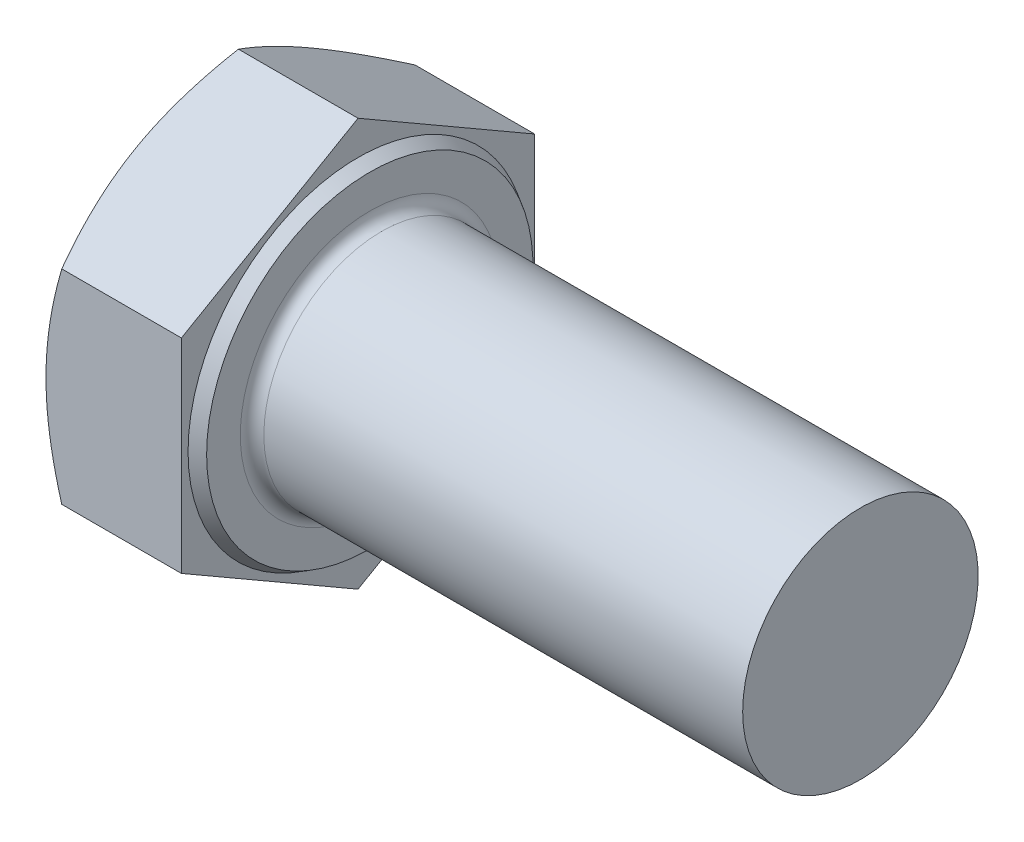
SolidWorks part; units mm, degrees
ref_plane "前视" through (0, 0, 0) normal (0, 0, 1) x (1, 0, 0)
ref_plane "上视" through (0, 0, 0) normal (0, 1, 0) x (1, 0, 0)
ref_plane "右视" through (0, 0, 0) normal (1, 0, 0) x (0, 0, -1)
sketch "草图1" plane through (0, 0, 0) normal (1, 0, 0) x (0, 0, -1)
  line L0 (9, 5.1962) -> (9, -5.1962)
  line L1 (-9, 5.1962) -> (-9, -5.1962)
  line L2 (9, -5.1962) -> (0, -10.3923)
  line L3 (0, -10.3923) -> (-9, -5.1962)
  line L4 (9, 5.1962) -> (0, 10.3923)
  line L5 (0, 10.3923) -> (-9, 5.1962)
  circle A0 centre (0, 0) radius 10.015 construction
  dimension "e" = 20.03
  dimension "s" = 18
  dimension "D2" = 120
  dimension "D3" = 9
  dimension "D4" = 9
  dimension "D5" = 9
extrude "基体-拉伸" add sketch "草图1" along normal blind 7.5
sketch "草图2" plane through (0, 0, 0) normal (0, 0, 1) x (1, 0, 0)
  line L0 (0, 5.1962) -> (0, -5.1962) construction
  line L1 (0, 0) -> (32.5, 0)
  line L2 (0, 0) -> (0, 6)
  line L3 (0, 6) -> (2.5, 6)
  line L4 (32.5, 0) -> (32.5, 4.4845)
  line L5 (7.5, 10.3923) -> (7.5, 5.1962) construction
  line L7 (0, 0) -> (44.5, 0) construction
  line L8 (32.5, -4.4845) -> (2.5, -6) construction
  line L9 (0, -6) -> (2.5, -6) construction
  line L10 (9.25, 6) -> (9.25, 0) construction
  line L11 (2.5, 15.24) -> (2.5, -1.27) construction
  line L12 (7.5, 5.1962) -> (7.5, -5.1962) construction
  line L13 (2.5, 6) -> (32.5, 6)
  line L14 (32.5, 6) -> (32.5, 4.4845)
  dimension "l" = 25
  dimension "d" = 12
  dimension "Minor_dia" = 8.969
  dimension "p" = 1.75
  dimension "b" = 30
  dimension "ds" = 12
revolve "凸台-旋转1" add sketch "草图2" angle 360 about L7
cosmetic thread "螺旋线1" parameters "Thread_length"=30, "Thread_minor"=8.969
sketch "草图3" plane through (0, 0, 0) normal (0, 0, 1) x (1, 0, 0)
  line L0 (0, 9) -> (3.6906, 15.3923)
  line L1 (0, 10.3923) -> (0, 5.1962) construction
  line L2 (3.6906, 15.3923) -> (3.6906, 20.3923)
  line L3 (3.6906, 20.3923) -> (-10, 20.3923)
  line L4 (-10, 20.3923) -> (-10, 9)
  line L5 (-10, 9) -> (0, 9)
  line L6 (0, 0) -> (99.06, 0) construction
  line L7 (7.5, 10.3923) -> (0, 10.3923) construction
  dimension "D1" = 9
  dimension "D2" = 5
  dimension "D3" = 10
  dimension "D4" = 5
  dimension "Head_ch_ang" = 30
revolve "切除-旋转1" cut sketch "草图3" angle 360 about L6
sketch "草图4" plane through (0, 0, 0) normal (0, 0, 1) x (1, 0, 0)
  line L0 (7.5, 0) -> (7.5, 8.315) construction
  line L2 (7.5, -6) -> (7.5, 6) construction
  line L3 (7.5, 10.3923) -> (7.5, 5.1962) construction
  line L4 (7.5, 8.315) -> (6.9, 8.6614)
  line L5 (0, 0) -> (95.25, 0) construction
  line L6 (0, 0) -> (44.5, 0) construction
  line L9 (6.9, 8.6614) -> (6.9, 10.3923)
  line L10 (7.5, 10.3923) -> (0.8038, 10.3923) construction
  line L11 (6.9, 10.3923) -> (7.5, 10.3923)
  line L12 (7.5, 10.3923) -> (7.5, 8.315)
  dimension "D1" = 120
  dimension "c" = 0.6
  dimension "dw" = 16.63
revolve "切除-旋转3" cut sketch "草图4" angle 360 about L5
fillet "圆角" radius 0.6 1 edges at (7.5, 0, -6)
sketch "草图6" plane through (0, 0, 0) normal (0, 0, 1) x (1, 0, 0)
  line L0 (0, 0) -> (32.5, 0) construction
  line L1 (32.5, -6) -> (32.5, 6) construction
  line L2 (32.5, 0) -> (32.5, 6) construction
  line L4 (31.625, 6) -> (33.375, 6)
  line L5 (31.625, 6) -> (32.5, 4.4845)
  line L6 (32.5, 4.4845) -> (33.375, 6)
  dimension "D1" = 1.75
revolve "切除-旋转4" [suppressed] cut sketch "草图6" angle 360 about L0
pattern_linear "阵列(线性)1" [suppressed]
